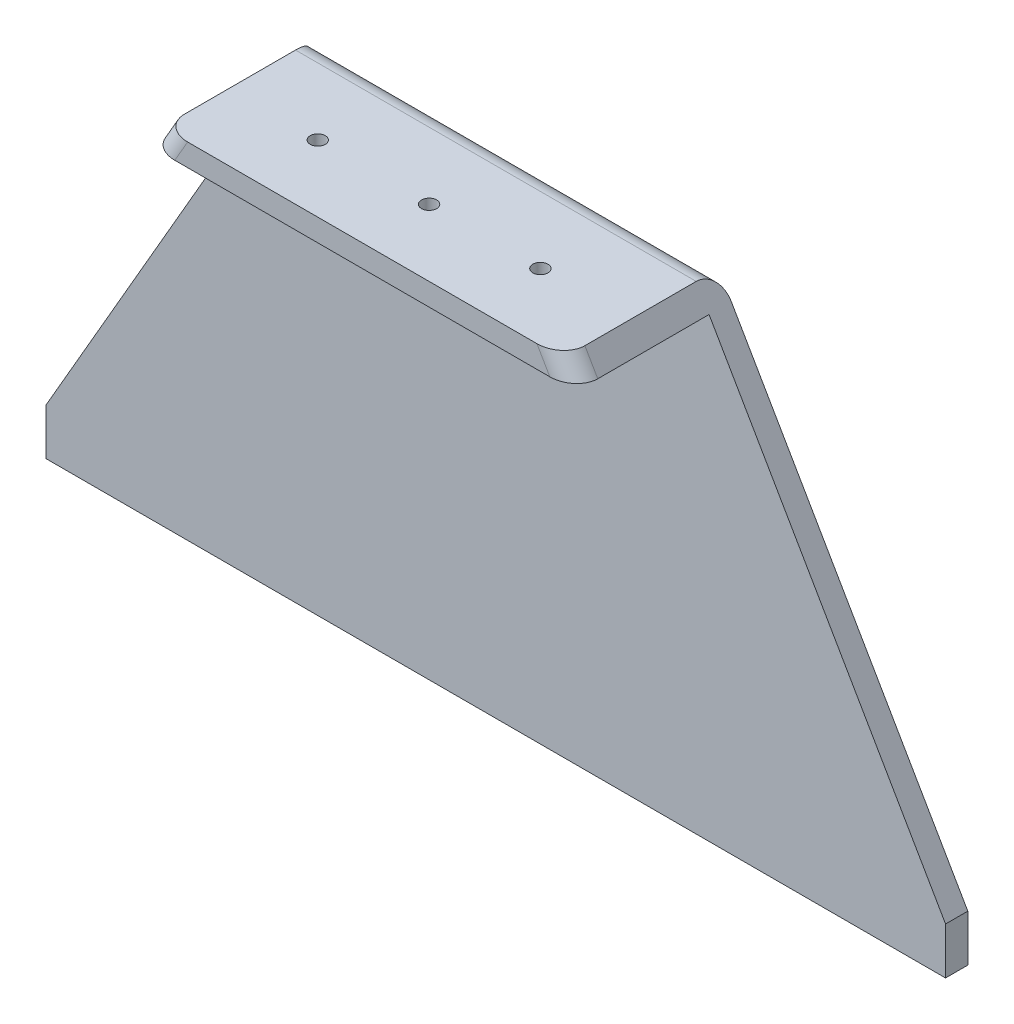
from build123d import *

# Parameters (mm, degrees)
SKETCH_1_W             = 404
SKETCH_1_H             = 215
EXTRUDE_1_DEPTH        = 70
SHELL_1_T              = -10
CUT_EXTRUDE_1_DEPTH    = 80
SKETCH_6_W             = 881.925411548
SKETCH_6_H             = 167.715249963
CUT_EXTRUDE_2_DEPTH    = 205
HOLE_WIZARD_M8_1_D     = 6.8
HOLE_WIZARD_M8_1_DEPTH = 19.75
HOLE_WIZARD_M8_1_TIP   = 2.042926105
FILLET_1_R             = 10


with BuildPart() as part:
    # 草图1 → 凸台-拉伸1 (new body)
    with BuildSketch(Plane.XY):
        Rectangle(SKETCH_1_W, SKETCH_1_H)
    extrude(amount=EXTRUDE_1_DEPTH)

    # 抽壳1
    shell_1_openings = [part.faces().sort_by_distance(p)[0] for p in [
        (-202, 0, 35),
        (202, 0, 35),
    ]]
    offset(amount=SHELL_1_T, openings=shell_1_openings, kind=Kind.INTERSECTION)

    # 草图2 → 切除-拉伸1 (cut)
    with BuildSketch(Plane.XY.offset(70)):
        Polygon((-202, -86.489690448), (-90, 107.5), (-202, 107.5), align=None)
        Polygon((90, 107.5), (202, 107.5), (202, -86.489690448), align=None)
    extrude(amount=-CUT_EXTRUDE_1_DEPTH, mode=Mode.SUBTRACT)

    # 草图6 → 切除-拉伸2 (cut)
    with BuildSketch(Plane.XZ.offset(107.5)):
        with Locations((-202, 93.857624982)):
            Rectangle(SKETCH_6_W, SKETCH_6_H)
    extrude(amount=-CUT_EXTRUDE_2_DEPTH, mode=Mode.SUBTRACT)

    # M8 螺纹孔1
    with Locations(Plane(origin=(0, 107.5, 0), x_dir=(1, 0, 0), z_dir=(0, 1, 0))):
        with Locations((-50, -40), (0, -40), (50, -40)):
            Hole(HOLE_WIZARD_M8_1_D / 2, depth=HOLE_WIZARD_M8_1_DEPTH)
            with Locations((0, 0, -(HOLE_WIZARD_M8_1_DEPTH + HOLE_WIZARD_M8_1_TIP / 2))):  # 118° drill point
                Cone(0, HOLE_WIZARD_M8_1_D / 2, HOLE_WIZARD_M8_1_TIP, mode=Mode.SUBTRACT)

    # 圆角1
    fillet_1_edges = [part.edges().sort_by_distance(p)[0] for p in [
        (0, 107.5, 0),
        (92.886751346, 102.5, 70),
        (-92.886751346, 102.5, 70),
    ]]
    fillet(fillet_1_edges, radius=FILLET_1_R)


solid = part.part
